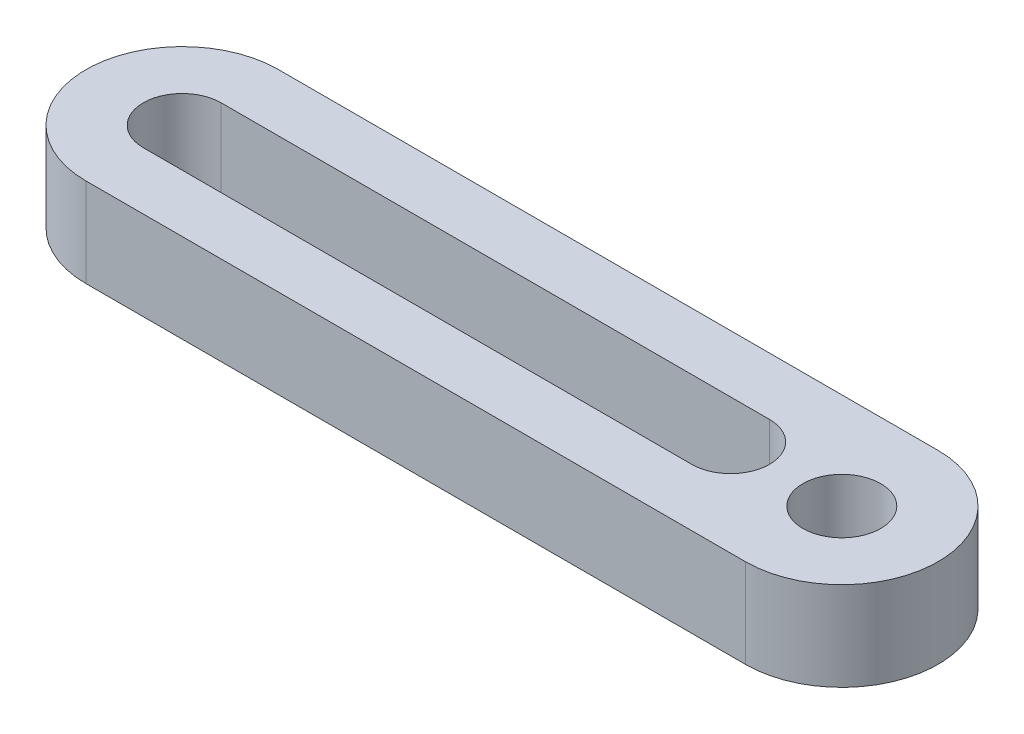
from build123d import *

# Parameters (mm, degrees)
SKETCH1_R           = 5.25
BOSS_EXTRUDE1_DEPTH = 6


with BuildPart() as part:
    # Sketch1 → Boss-Extrude1 (new, symmetric)
    with BuildSketch(Plane(origin=(0, 0, 0), x_dir=(1, 0, 0), z_dir=(0, 1, 0))):
        with BuildLine():
            Line((-44.5, 13), (44.5, 13))
            ThreePointArc((44.5, 13), (57.5, 0), (44.5, -13))
            Line((44.5, -13), (-44.5, -13))
            ThreePointArc((-44.5, -13), (-57.5, 0), (-44.5, 13))
        make_face()
        with Locations(Location((44.5, 0, 0), (0, 0, 270))):
            Circle(SKETCH1_R, mode=Mode.SUBTRACT)
        with BuildLine():
            Line((-44.5, 5.25), (29.5, 5.25))
            ThreePointArc((29.5, 5.25), (34.75, 0), (29.5, -5.25))
            Line((29.5, -5.25), (-44.5, -5.25))
            ThreePointArc((-44.5, -5.25), (-49.75, 0), (-44.5, 5.25))
        make_face(mode=Mode.SUBTRACT)
    extrude(amount=BOSS_EXTRUDE1_DEPTH, both=True)


solid = part.part
